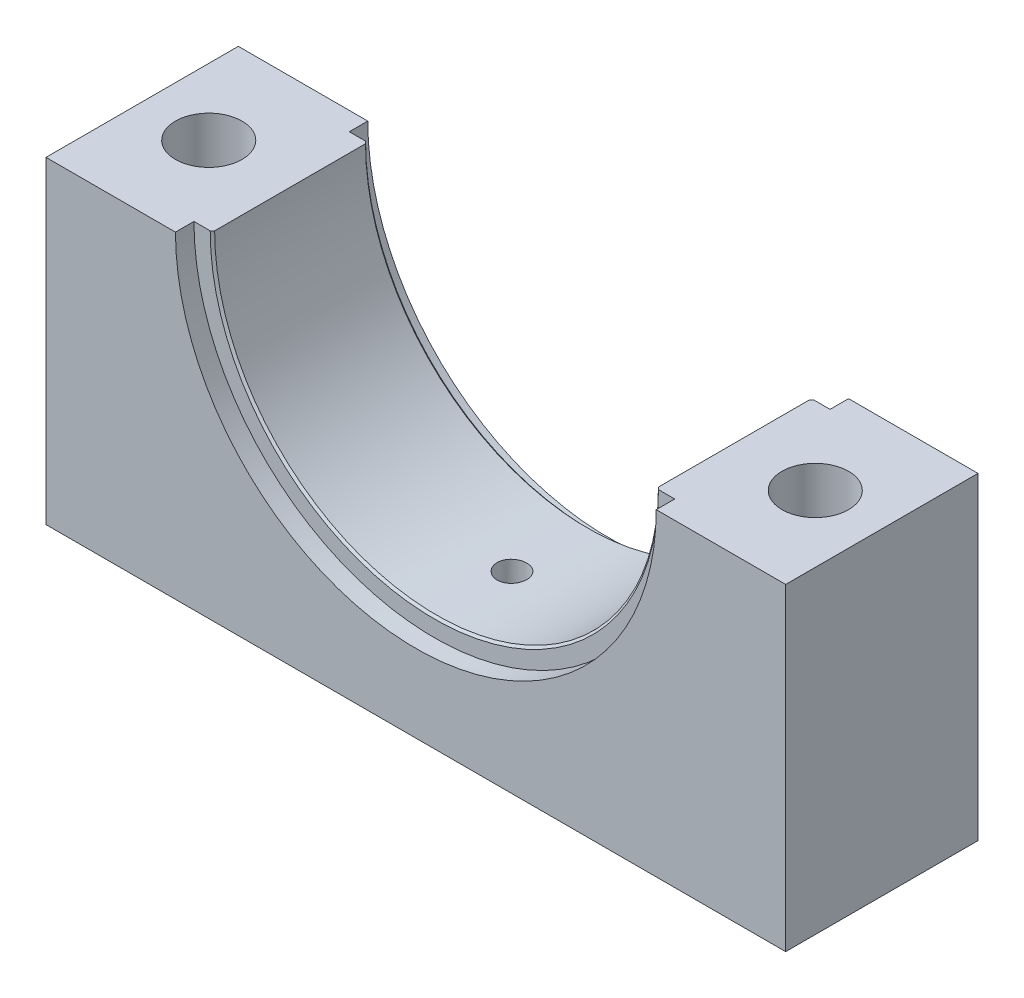
from build123d import *

# Parameters (mm, degrees)
BOSS_EXTRUDE1_DEPTH = 26
SKETCH2_R           = 32.5
CUT_EXTRUDE1_DEPTH  = 2.5
CUT_EXTRUDE2_START  = -2.5
SKETCH3_R           = 32.5
CUT_EXTRUDE2_DEPTH  = 2.5
CHAMFER1_SIZE       = 0.3
HOLE1_D             = 9
HOLE2_D             = 4
HOLE2_DEPTH         = 34
HOLE4_D             = 8
HOLE4_DEPTH         = 6
CUT_EXTRUDE4_DEPTH  = 6


with BuildPart() as part:
    # Sketch1 → Boss-Extrude1 (new body)
    with BuildSketch(Plane.XY):
        with BuildLine():
            Line((-50, 0), (-30, 0))
            ThreePointArc((-30, 0), (0, -30), (30, 0))
            Line((30, 0), (50, 0))
            Line((50, 0), (50, -43))
            Line((50, -43), (-50, -43))
            Line((-50, -43), (-50, 0))
        make_face()
    extrude(amount=BOSS_EXTRUDE1_DEPTH)

    # Sketch2 → Cut-Extrude1 (cut)
    with BuildSketch(Plane.XY.offset(26)):
        Circle(SKETCH2_R)
    extrude(amount=-CUT_EXTRUDE1_DEPTH, mode=Mode.SUBTRACT)

    # Sketch3 → Cut-Extrude2 (cut)
    with BuildSketch(Plane(origin=(0, 0, 0), x_dir=(-1, 0, 0), z_dir=(0, 0, -1)).offset(CUT_EXTRUDE2_START)):
        Circle(SKETCH3_R)
    extrude(amount=CUT_EXTRUDE2_DEPTH, mode=Mode.SUBTRACT)

    # Chamfer1
    chamfer1_edges = [part.edges().sort_by_distance(p)[0] for p in [
        (0, -30, 23.5),
        (0, -30, 2.5),
    ]]
    chamfer(chamfer1_edges, length=CHAMFER1_SIZE)

    # Hole1 (through all)
    with Locations(Plane(origin=(0, 0, 0), x_dir=(1, 0, 0), z_dir=(0, 1, 0))):
        with Locations((-41, -13), (41, -13)):
            Hole(HOLE1_D / 2)

    # Hole2
    with Locations(Plane(origin=(0, 0, 0), x_dir=(1, 0, 0), z_dir=(0, 1, 0))):
        with Locations((0, -13)):
            Hole(HOLE2_D / 2, depth=HOLE2_DEPTH)

    # Hole4
    with Locations(Plane(origin=(0, -43, 0), x_dir=(-1, 0, 0), z_dir=(0, -1, 0))):
        with Locations((-21, -13)):
            Hole(HOLE4_D / 2, depth=HOLE4_DEPTH)

    # Sketch11 → Cut-Extrude4 (cut)
    with BuildSketch(Plane.XZ.offset(43)):
        with BuildLine():
            Line((-20, 17), (-22, 17))
            ThreePointArc((-22, 17), (-26, 13), (-22, 9))
            Line((-22, 9), (-20, 9))
            ThreePointArc((-20, 9), (-16, 13), (-20, 17))
        make_face()
    extrude(amount=-CUT_EXTRUDE4_DEPTH, mode=Mode.SUBTRACT)


solid = part.part
